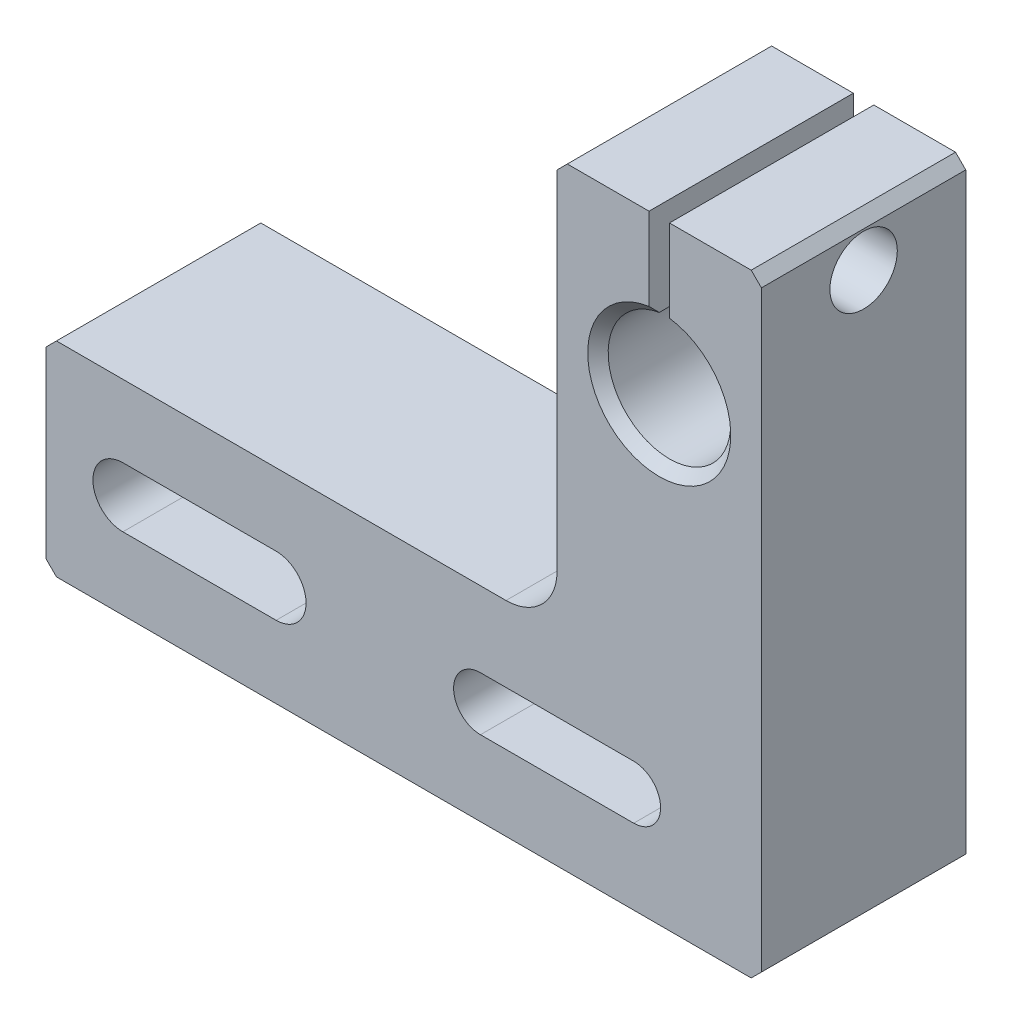
SolidWorks part; units mm, degrees
material "Q235-A"
ref_plane "Front Plane" through (0, 0, 0) normal (0, 0, 1) x (1, 0, 0)
ref_plane "Top Plane" through (0, 0, 0) normal (0, 1, 0) x (1, 0, 0)
ref_plane "Right Plane" through (0, 0, 0) normal (1, 0, 0) x (0, 0, -1)
sketch "Sketch1" plane through (0, 0, 0) normal (0, 0, 1) x (1, 0, 0)
  line L0 (22.0499, 34.7959) -> (22.0499, -25.2041)
  line L1 (22.0499, -25.2041) -> (-47.9501, -25.2041)
  line L2 (-47.9501, -25.2041) -> (-47.9501, -5.2041)
  line L3 (-47.9501, -5.2041) -> (2.0499, -5.2041)
  line L4 (2.0499, -5.2041) -> (2.0499, 34.7959)
  line L5 (2.0499, 34.7959) -> (11.0499, 34.7959)
  line L6 (-40.4501, -15.2041) -> (-25.4501, -15.2041) construction
  line L7 (-40.4501, -12.275) -> (-25.4501, -12.275)
  line L8 (-40.4501, -18.1331) -> (-25.4501, -18.1331)
  line L9 (-5.4501, -15.2041) -> (9.5499, -15.2041) construction
  line L10 (-5.4501, -12.5761) -> (9.5499, -12.5761)
  line L11 (-5.4501, -17.8321) -> (9.5499, -17.8321)
  line L12 (13.0499, 34.7959) -> (22.0499, 34.7959)
  line L14 (11.0499, 34.7959) -> (11.0499, 25.712)
  line L16 (13.0499, 34.7959) -> (13.0499, 25.712)
  arc A0 (-40.4501, -12.275) -> (-40.4501, -18.1331) centre (-40.4501, -15.2041) ccw
  arc A1 (-25.4501, -18.1331) -> (-25.4501, -12.275) centre (-25.4501, -15.2041) ccw
  arc A2 (-5.4501, -12.5761) -> (-5.4501, -17.8321) centre (-5.4501, -15.2041) ccw
  arc A3 (9.5499, -17.8321) -> (9.5499, -12.5761) centre (9.5499, -15.2041) ccw
  arc A4 (11.0499, 25.712) -> (13.0499, 25.712) centre (12.0499, 19.7959) ccw
  point P8 (-32.9501, -15.2041)
  point P13 (2.0499, -15.2041)
  point P22 (12.0499, 34.7959)
  dimension "D10" = 45
  dimension "D11" = 10
  dimension "D12" = 12
  dimension "D1" = 20
  dimension "D2" = 60
  dimension "D3" = 70
  dimension "D4" = 20
  dimension "D5" = 15
  dimension "D6" = 15
  dimension "D7" = 35
  dimension "D8" = 7.5
  dimension "D9" = 10
extrude "Boss-Extrude1" add sketch "Sketch1" along normal blind 20
chamfer "Chamfer1" distance 1 angle 45 2 edges at (12.0499, 13.7959, 0) (12.0499, 13.7959, 20)
sketch "Sketch2" plane through (2.0499, 0, 0) normal (-1, 0, 0) x (0, 0, 1)
  line L1 (20, -25.2041) -> (0, -25.2041) construction
  circle A0 centre (10, 30.2959) radius 2.0281
  dimension "D1" = 55.5
hole_wizard "M6 Tapped Hole1" positions "Sketch3" profile "Sketch4" tap size "M6" standard "GB"
sketch "Sketch3" plane through (2.0499, 0, 0) normal (-1, 0, 0) x (0, 0, 1)
  point P2 (10, 30.2959)
cosmetic thread "Cosmetic thread 1" parameters "D1"=9, "D2"=6
sketch "Sketch4" plane through (2.0499, 30.2959, 10) normal (0, 1, 0) x (0, 0, 1)
  line L0 (0, 0) -> (0, 10.5022)
  line L1 (0, 10.5022) -> (2.5, 9)
  line L2 (2.5, 9) -> (2.5, 0)
  line L5 (2.5, 0) -> (0, 0)
  line L10 (0, 10.5022) -> (-2.5, 9) construction
  line L11 (0, -6.35) -> (0, 107.95) construction
  dimension "螺纹孔钻头直径" = 5
  dimension "螺纹孔钻头深度" = 9
  dimension "导头角度" = 118
sketch "Sketch5" plane through (22.0499, 0, 0) normal (1, 0, 0) x (0, 0, -1)
  line L0 (-20, -25.2041) -> (0, -25.2041) construction
  circle A0 centre (-10, 30.2959) radius 2.6347
  dimension "D1" = 55.5
hole_wizard "Hole1" positions "Sketch6" profile "Sketch7" legacy
sketch "Sketch6" plane through (22.0499, 0, 0) normal (1, 0, 0) x (0, 0, -1)
  point P0 (-10, 30.2959)
sketch "Sketch7" plane through (22.0499, 30.2959, 10) normal (0, 1, 0) x (0, 0, -1)
  line L0 (0, 0) -> (0, 9)
  line L1 (0, 9) -> (3.3, 9)
  line L2 (3.3, 9) -> (3.3, 0)
  line L3 (3.3, 0) -> (0, 0)
  line L4 (0, 110) -> (0, -10) construction
  dimension "直径" = 6.6
  dimension "深度" = 9
chamfer "Chamfer2" distance 1 angle 45 5 edges at (-47.9501, -25.2041, 10) (-47.9501, -5.2041, 10) (22.0499, -25.2041, 10) (2.0499, 34.7959, 10) (22.0499, 34.7959, 10)
fillet "Fillet1" radius 5 1 edges at (2.0499, -5.2041, 10)
